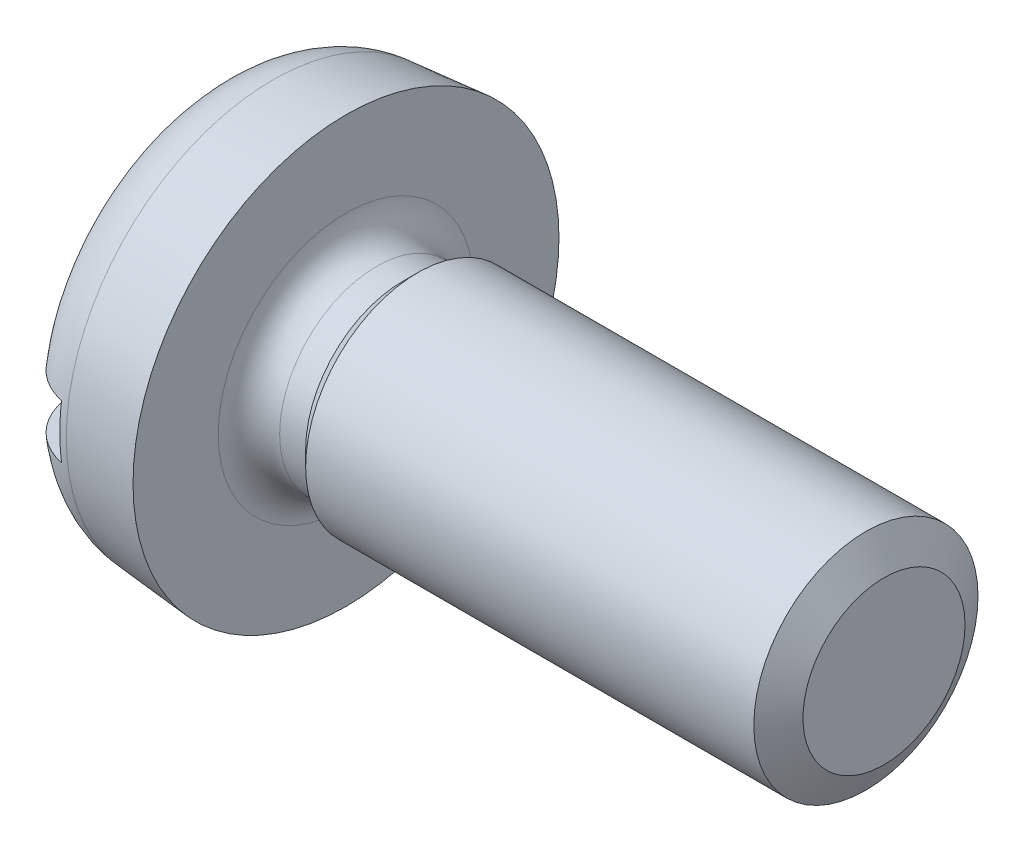
from build123d import *

# Parameters (mm, degrees)
SKETCH4_W          = 1.2
SKETCH4_H          = 1.2
CUT_EXTRUDE1_DEPTH = 50


with BuildPart() as part:
    # Sketch3 → Boss-Revolve (revolve)
    with BuildSketch(Plane.XY, mode=Mode.PRIVATE) as boss_revolve_sk:
        with BuildLine():
            Line((0, 0), (15, 0))
            Line((15, 0), (15, 2.5))
            Line((15, 2.5), (4.6, 2.5))
            Line((4.6, 2.5), (4.265, 2.165))
            Line((4.265, 2.165), (3.685, 2.165))
            ThreePointArc((3.685, 2.165), (3.200631855, 2.365631855), (3, 2.85))
            Line((3, 2.85), (3, 4.75))
            Line((3, 4.75), (1.369266386, 4.607329296))
            ThreePointArc((1.369266386, 4.607329296), (0.394083995, 4.12642256), (0, 3.113037248))
            Line((0, 3.113037248), (0, 0))
        make_face()
    revolve(boss_revolve_sk.sketch.rotate(Axis((-2.477021524, 0, 0), (1, 0, 0)), 90), axis=Axis((-2.477021524, 0, 0), (1, 0, 0)))

    # Sketch4 → Cut-Extrude1 (cut, symmetric)
    with BuildSketch(Plane.XY):
        with Locations((0.6, 0)):
            Rectangle(SKETCH4_W, SKETCH4_H)
    extrude(amount=CUT_EXTRUDE1_DEPTH, both=True, mode=Mode.SUBTRACT)

    # Sketch5 → Cut-Revolve1 (revolve, cut)
    with BuildSketch(Plane.XY, mode=Mode.PRIVATE) as cut_revolve1_sk:
        Polygon((14.595667195, 2.5), (15.395667195, 2.5), (15, 1.8072), align=None)
    revolve(cut_revolve1_sk.sketch.rotate(Axis((6.174994867, 0, 0), (-1, 0, 0)), 270), axis=Axis((6.174994867, 0, 0), (-1, 0, 0)), mode=Mode.SUBTRACT)


solid = part.part
